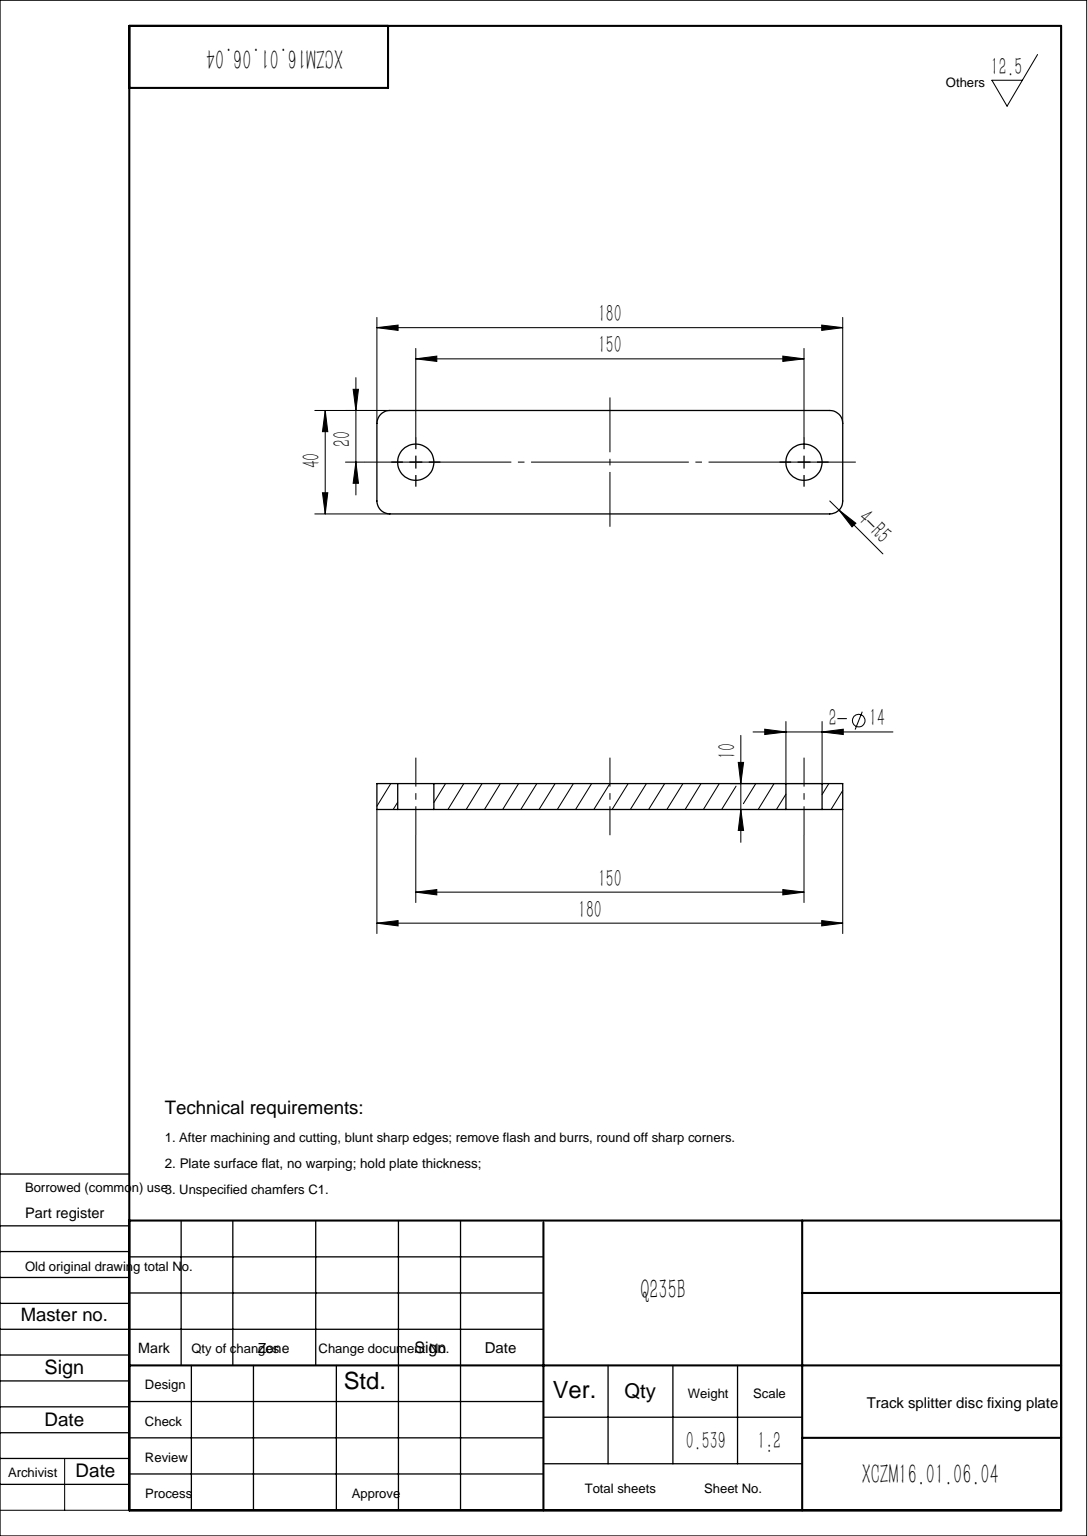
SolidWorks part; units mm, degrees
material "Q235B"
ref_plane "Front Plane" through (0, 0, 0) normal (0, 0, 1) x (1, 0, 0)
ref_plane "Top Plane" through (0, 0, 0) normal (0, 1, 0) x (1, 0, 0)
ref_plane "Right Plane" through (0, 0, 0) normal (1, 0, 0) x (0, 0, -1)
sketch "Sketch2" plane through (0, 0, 0) normal (0, 1, 0) x (1, 0, 0)
  line L0 (0, 20) -> (0, -20) construction
  line L1 (85, -20) -> (-85, -20)
  line L2 (90, -15) -> (90, 15)
  line L3 (85, 20) -> (-85, 20)
  line L4 (-90, -15) -> (-90, 15)
  line L5 (90, -20) -> (-90, 20) construction
  line L6 (90, 20) -> (-90, -20) construction
  arc A0 (-85, -20) -> (-90, -15) centre (-85, -15) cw
  arc A1 (90, 15) -> (85, 20) centre (85, 15) ccw
  arc A2 (85, -20) -> (90, -15) centre (85, -15) ccw
  arc A3 (-85, 20) -> (-90, 15) centre (-85, 15) ccw
  circle A4 centre (-75, 0) radius 7
  circle A5 centre (75, 0) radius 7
  point P0 (0, 0)
  dimension "D3" = 5
  dimension "D4" = 14
  dimension "D5" = 150
  dimension "D1" = 40
  dimension "D2" = 180
extrude "Boss-Extrude1" add sketch "Sketch2" along normal blind 10
